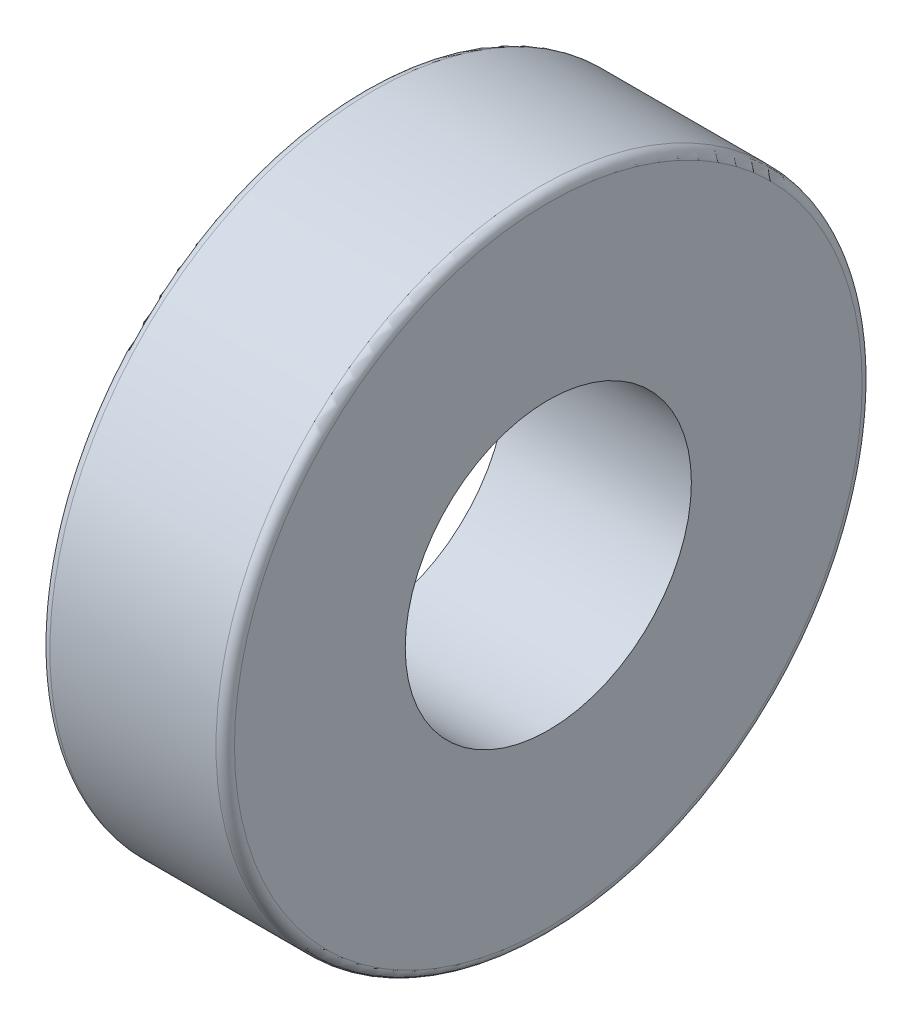
SolidWorks part; units mm, degrees
ref_plane "前视基准面" through (0, 0, 0) normal (0, 0, 1) x (1, 0, 0)
ref_plane "上视基准面" through (0, 0, 0) normal (0, 1, 0) x (1, 0, 0)
ref_plane "右视基准面" through (0, 0, 0) normal (1, 0, 0) x (0, 0, -1)
sketch "草图1" plane through (0, 0, 0) normal (0, 0, 1) x (1, 0, 0)
  line L0 (-20, 0) -> (20, 0) construction
  line L1 (-20, 70) -> (-20, 0)
  line L2 (20, 70) -> (20, 0)
  line L3 (20, 0) -> (-20, 0)
  line L4 (-20, 70) -> (20, 70)
  point P6 (0, 0)
  dimension "D1" = 40
  dimension "D2" = 70
revolve "旋转1" add sketch "草图1" angle 360 about L0
sketch "草图2" plane through (20, 0, 0) normal (1, 0, 0) x (0, 0, -1)
  circle A0 centre (0, 0) radius 31
  dimension "D1" = 62
extrude "切除-拉伸1" cut sketch "草图2" against normal through all
fillet "圆角1" radius 2 2 edges at (20, -70, 0) (-20, -70, 0)
